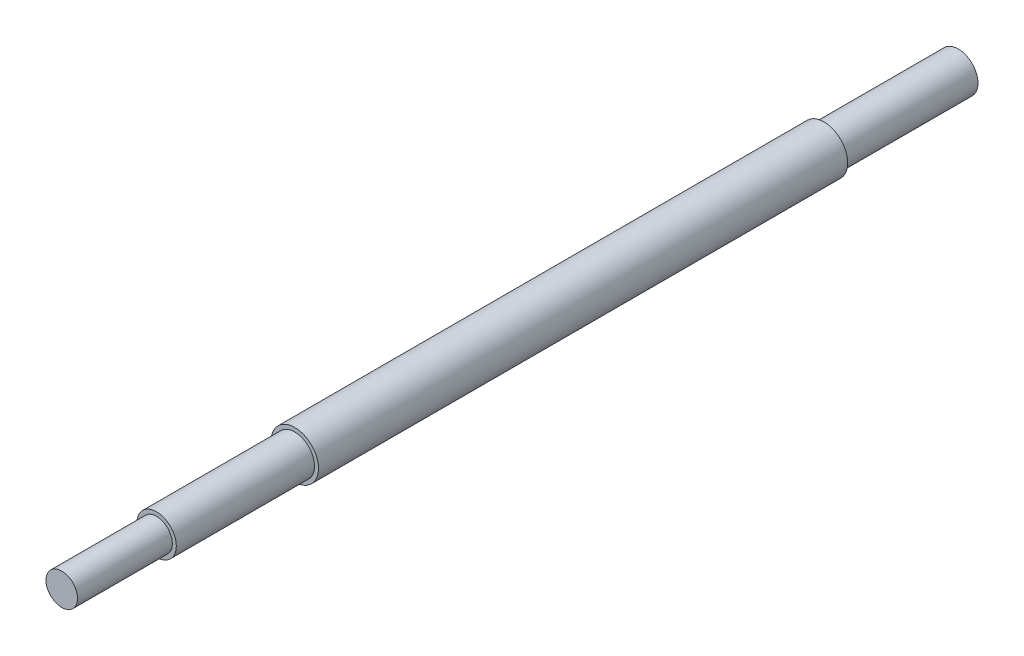
from build123d import *

# Parameters (mm, degrees)
SKETCH1_R           = 2.5
BOSS_EXTRUDE1_DEPTH = 17
SKETCH2_R           = 3
BOSS_EXTRUDE2_DEPTH = 67
SKETCH3_R           = 2.5
BOSS_EXTRUDE3_DEPTH = 17.5
SKETCH4_R           = 2
BOSS_EXTRUDE4_DEPTH = 12


with BuildPart() as part:
    # Sketch1 → Boss-Extrude1 (new body)
    with BuildSketch(Plane.XY):
        Circle(SKETCH1_R)
    extrude(amount=BOSS_EXTRUDE1_DEPTH)

    # Sketch2 → Boss-Extrude2 (add)
    with BuildSketch(Plane.XY.offset(17)):
        Circle(SKETCH2_R)
    extrude(amount=BOSS_EXTRUDE2_DEPTH)

    # Sketch3 → Boss-Extrude3 (add)
    with BuildSketch(Plane.XY.offset(84)):
        Circle(SKETCH3_R)
    extrude(amount=BOSS_EXTRUDE3_DEPTH)

    # Sketch4 → Boss-Extrude4 (add)
    with BuildSketch(Plane.XY.offset(101.5)):
        Circle(SKETCH4_R)
    extrude(amount=BOSS_EXTRUDE4_DEPTH)


solid = part.part
